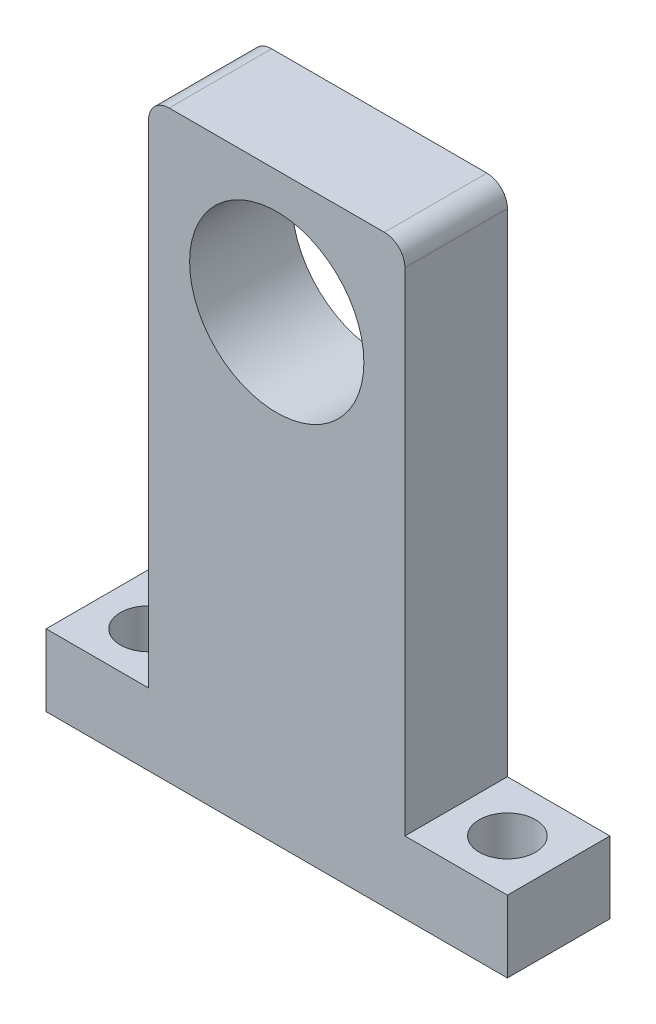
from build123d import *

# Parameters (mm, degrees)
SKETCH_1_R          = 8.5
EXTRUDE_1_DEPTH     = 5
FILLET_1_R          = 2
CUT_EXTRUDE_1_REACH = 57.057
SKETCH_2_R          = 2.75


with BuildPart() as part:
    # 草图1 → 凸台-拉伸1 (new, symmetric)
    with BuildSketch(Plane.XY):
        Polygon((0, 0), (-22.5, 0), (-22.5, 7), (-12.5, 7), (-12.5, 57), (12.5, 57), (12.5, 7), (22.5, 7), (22.5, 0), align=None)
        with Locations((0, 45)):
            Circle(SKETCH_1_R, mode=Mode.SUBTRACT)
    extrude(amount=EXTRUDE_1_DEPTH, both=True)

    # 圆角1
    fillet_1_edges = [part.edges().sort_by_distance(p)[0] for p in [
        (-12.5, 57, 0),
        (12.5, 57, 0),
    ]]
    fillet(fillet_1_edges, radius=FILLET_1_R)

    # 草图2 → 切除-拉伸1 (cut, up to next)
    with BuildSketch(Plane(origin=(0, 7, 0), x_dir=(1, 0, 0), z_dir=(0, 1, 0)), mode=Mode.PRIVATE) as cut_extrude_1_sk1:
        with Locations(Location((-17.5, 0, 0), (0, 0, 180))):
            Circle(SKETCH_2_R)
    cut_extrude_1_tool1 = extrude(cut_extrude_1_sk1.sketch, amount=-CUT_EXTRUDE_1_REACH, mode=Mode.PRIVATE) & part.part
    # 草图2 → 切除-拉伸1 (cut, up to next)
    with BuildSketch(Plane(origin=(0, 7, 0), x_dir=(1, 0, 0), z_dir=(0, 1, 0)), mode=Mode.PRIVATE) as cut_extrude_1_sk2:
        with Locations(Location((17.5, 0, 0), (0, 0, 180))):
            Circle(SKETCH_2_R)
    cut_extrude_1_tool2 = extrude(cut_extrude_1_sk2.sketch, amount=-CUT_EXTRUDE_1_REACH, mode=Mode.PRIVATE) & part.part
    add(cut_extrude_1_tool1.solids().sort_by_distance((-17.5, 7, 0))[0], mode=Mode.SUBTRACT)
    add(cut_extrude_1_tool2.solids().sort_by_distance((17.5, 7, 0))[0], mode=Mode.SUBTRACT)


solid = part.part
